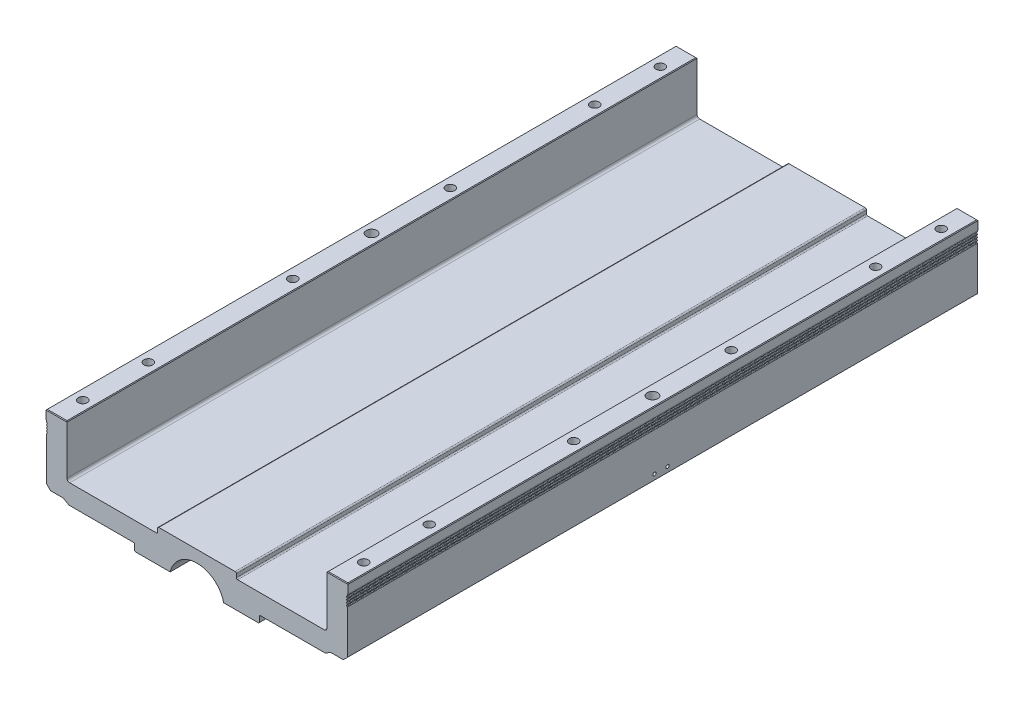
from build123d import *

# Parameters (mm, degrees)
EXTRUDE_1_DEPTH             = 240
CUT_EXTRUDE_1_DEPTH         = 504.178149367
FILLET_1_R                  = 2
FILLET_8_R                  = 1
CUT_EXTRUDE_3_DEPTH         = 504.178149367
FILLET_6_R                  = 0.5
CUT_EXTRUDE_4_DEPTH         = 504.178149367
SKETCH_8_W                  = 1.5
SKETCH_8_H                  = 10.5
CUT_EXTRUDE_6496_DEPTH      = 504.178149367
SKETCH_9_W                  = 230
SKETCH_9_H                  = 1.5
CUT_EXTRUDE_6896_DEPTH      = 503.832974257
SKETCH_10_W                 = 67
SKETCH_10_H                 = 5.5
CUT_EXTRUDE_7625_DEPTH      = 503.832974257
SKETCH_31_W                 = 27
SKETCH_31_H                 = 3
CUT_EXTRUDE_10_DEPTH        = 503.832974257
HOLE_WIZARD_M8_1_D          = 6.8
HOLE_WIZARD_M8_1_DEPTH      = 26.25
HOLE_WIZARD_M8_1_TIP        = 2.042926105
SKETCH_22_R                 = 4
CUT_EXTRUDE_8_DEPTH         = 15
HOLE_WIZARD_M3_1_AT_2_COUNT = 2
HOLE_WIZARD_M3_1_AT_2_PITCH = 10
CHAMFER_3_SIZE              = 0.5
SKETCH_30_R                 = 5
CUT_EXTRUDE_9_DEPTH         = 6
SKETCH_32_W                 = 66
SKETCH_32_H                 = 34.5
CUT_EXTRUDE_11_DEPTH        = 503.832974257


with BuildPart() as part:
    # 草图1 → 凸台-拉伸1 (new, symmetric)
    with BuildSketch(Plane.XY):
        Polygon((-116.5, 0), (116.5, 0), (116.5, -8), (116, -8.5), (114.5, -8.5), (114.5, -50.5), (111.5, -53.5), (101.92820323, -53.5), (95, -57.5), (49, -57.5), (49, -59.5), (47, -61.5), (33, -61.5), (33, -86), (27.226497308, -96), (-27.226497308, -96), (-33, -86), (-33, -61.5), (-47, -61.5), (-49, -59.5), (-49, -57.5), (-95, -57.5), (-101.92820323, -53.5), (-111.5, -53.5), (-114.5, -50.5), (-114.5, -8.5), (-116, -8.5), (-116.5, -8), align=None)
    extrude(amount=EXTRUDE_1_DEPTH, both=True)

    # 草图2 → 切除-拉伸1 (cut, through all)
    with BuildSketch(Plane.XY.offset(240)):
        Polygon((-99, 0), (99, 0), (99, -41), (30, -41), (30, -36.5), (-30, -36.5), (-30, -41), (-99, -41), align=None)
    extrude(amount=-CUT_EXTRUDE_1_DEPTH, mode=Mode.SUBTRACT)

    # 圆角1
    fillet_1_edges = [part.edges().sort_by_distance(p)[0] for p in [
        (99, -41, 0),
        (-99, -41, 0),
    ]]
    fillet(fillet_1_edges, radius=FILLET_1_R)

    # 圆角8
    fillet_8_edges = [part.edges().sort_by_distance(p)[0] for p in [
        (30, -41, 0),
        (30, -36.5, 0),
        (-30, -36.5, 0),
        (-30, -41, 0),
    ]]
    fillet(fillet_8_edges, radius=FILLET_8_R)

    # 草图4 → 切除-拉伸3 (cut, through all)
    with BuildSketch(Plane.XY.offset(240)):
        with BuildLine():
            Line((-114.5, -10), (-114.5, -11))
            ThreePointArc((-114.5, -11), (-114, -10.5), (-114.5, -10))
        make_face()
        with BuildLine():
            Line((-114.5, -12), (-114.5, -13))
            ThreePointArc((-114.5, -13), (-114, -12.5), (-114.5, -12))
        make_face()
        with BuildLine():
            Line((-114.5, -14), (-114.5, -15))
            ThreePointArc((-114.5, -15), (-114, -14.5), (-114.5, -14))
        make_face()
        with BuildLine():
            Line((-114.5, -16), (-114.5, -17))
            ThreePointArc((-114.5, -17), (-114, -16.5), (-114.5, -16))
        make_face()
        with BuildLine():
            Line((114.5, -16), (114.5, -17))
            ThreePointArc((114.5, -17), (114, -16.5), (114.5, -16))
        make_face()
        with BuildLine():
            Line((114.5, -14), (114.5, -15))
            ThreePointArc((114.5, -15), (114, -14.5), (114.5, -14))
        make_face()
        with BuildLine():
            Line((114.5, -12), (114.5, -13))
            ThreePointArc((114.5, -13), (114, -12.5), (114.5, -12))
        make_face()
        with BuildLine():
            Line((114.5, -10), (114.5, -11))
            ThreePointArc((114.5, -11), (114, -10.5), (114.5, -10))
        make_face()
    extrude(amount=-CUT_EXTRUDE_3_DEPTH, mode=Mode.SUBTRACT)

    # 圆角6
    fillet_6_edges = [part.edges().sort_by_distance(p)[0] for p in [
        (-114.5, -14, 0),
        (-114.5, -15, 0),
        (-114.5, -12, 0),
        (-114.5, -13, 0),
        (-114.5, -16, 0),
        (-114.5, -17, 0),
        (-114.5, -10, 0),
        (-114.5, -11, 0),
        (114.5, -13, 0),
        (114.5, -12, 0),
        (114.5, -11, 0),
        (114.5, -10, 0),
        (114.5, -15, 0),
        (114.5, -14, 0),
        (114.5, -17, 0),
        (114.5, -16, 0),
    ]]
    fillet(fillet_6_edges, radius=FILLET_6_R)

    # 草图5 → 切除-拉伸4 (cut, through all)
    with BuildSketch(Plane.XY.offset(240)):
        with BuildLine():
            Line((-13.5, -82.585707942), (-13.5, -93))
            Line((-13.5, -93), (13.5, -93))
            Line((13.5, -93), (13.5, -82.585707942))
            ThreePointArc((13.5, -82.585707942), (0, -45.5), (-13.5, -82.585707942))
        make_face()
    extrude(amount=-CUT_EXTRUDE_4_DEPTH, mode=Mode.SUBTRACT)

    # 草图8 → Cut-Extrude 6496 (cut, through all)
    with BuildSketch(Plane.XY.offset(240)):
        with Locations((115.75, -5.25)):
            Rectangle(SKETCH_8_W, SKETCH_8_H)
        with Locations((-115.75, -5.25)):
            Rectangle(SKETCH_8_W, SKETCH_8_H)
    extrude(amount=-CUT_EXTRUDE_6496_DEPTH, mode=Mode.SUBTRACT)

    # 草图9 → Cut-Extrude 6896 (cut, through all)
    with BuildSketch(Plane.XY.offset(240)):
        with Locations((0, -0.75)):
            Rectangle(SKETCH_9_W, SKETCH_9_H)
    extrude(amount=-CUT_EXTRUDE_6896_DEPTH, mode=Mode.SUBTRACT)

    # 草图10 → Cut-Extrude 7625 (cut, through all)
    with BuildSketch(Plane.XY.offset(240)):
        with Locations((81, -58.75)):
            Rectangle(SKETCH_10_W, SKETCH_10_H)
        with Locations((-81, -58.75)):
            Rectangle(SKETCH_10_W, SKETCH_10_H)
    extrude(amount=-CUT_EXTRUDE_7625_DEPTH, mode=Mode.SUBTRACT)

    # 草图31 → 切除-拉伸10 (cut, through all)
    with BuildSketch(Plane.XY.offset(240)):
        with Locations((0, -94.5)):
            Rectangle(SKETCH_31_W, SKETCH_31_H)
    extrude(amount=-CUT_EXTRUDE_10_DEPTH, mode=Mode.SUBTRACT)

    # M8 螺纹孔1
    with Locations(Plane(origin=(0, -1.5, 0), x_dir=(1, 0, 0), z_dir=(0, 1, 0))):
        with Locations((-107, 60), (-107, -60), (107, -60), (107, 60), (107, 220), (107, -220), (-107, -220), (-107, 220), (107, 170), (107, -170), (-107, -170), (-107, 170)):
            Hole(HOLE_WIZARD_M8_1_D / 2, depth=HOLE_WIZARD_M8_1_DEPTH)
            with Locations((0, 0, -(HOLE_WIZARD_M8_1_DEPTH + HOLE_WIZARD_M8_1_TIP / 2))):  # 118° drill point
                Cone(0, HOLE_WIZARD_M8_1_D / 2, HOLE_WIZARD_M8_1_TIP, mode=Mode.SUBTRACT)

    # 草图22 → 切除-拉伸8 (cut)
    with BuildSketch(Plane(origin=(0, -1.5, 0), x_dir=(1, 0, 0), z_dir=(0, 1, 0))):
        with Locations(Location((-107, 0, 0), (0, 0, 180))):
            Circle(SKETCH_22_R)
        with Locations(Location((107, 0, 0), (0, 0, 180))):
            Circle(SKETCH_22_R)
    extrude(amount=-CUT_EXTRUDE_8_DEPTH, mode=Mode.SUBTRACT)

    # 草图28 → M3 螺纹孔1 (revolve, cut)
    with BuildSketch(Plane(origin=(114.5, -46.5, -4), x_dir=(0, 0, -1), z_dir=(0, 1, 0))):
        Polygon((0, 0), (0, 9.251075774), (1.25, 8.5), (1.25, 0), align=None)
    hole_wizard_m3_1 = revolve(axis=Axis((120.85, -46.5, -4), (-1, 0, 0)), mode=Mode.SUBTRACT)

    # M3 螺纹孔1 at 2: M3 螺纹孔1 ×2
    with Locations(*[(0, 0, i * HOLE_WIZARD_M3_1_AT_2_PITCH) for i in range(1, HOLE_WIZARD_M3_1_AT_2_COUNT)]):
        add(hole_wizard_m3_1, mode=Mode.SUBTRACT)

    # 镜向1: M3 螺纹孔1 across plane
    add(hole_wizard_m3_1.mirror(Plane(origin=(0, 0, 0), x_dir=(0, 0, 1), z_dir=(1, 0, 0))), mode=Mode.SUBTRACT)

    # 镜向1 copy 1 sketch → 镜向1 copy 1 (revolve, cut)
    with BuildSketch(Plane(origin=(-114.5, -46.5, 6), x_dir=(0, 0, -1), z_dir=(0, 1, 0))):
        Polygon((0, 0), (0, -9.251075774), (1.25, -8.5), (1.25, 0), align=None)
    revolve(axis=Axis((-120.85, -46.5, 6), (-1, 0, 0)), mode=Mode.SUBTRACT)

    # 倒角3
    chamfer_3_edges = [part.edges().sort_by_distance(p)[0] for p in [
        (99, -1.5, 0),
        (107, -1.5, -240),
        (115, -1.5, 0),
        (-107, -1.5, -240),
        (-99, -1.5, 0),
        (107, -1.5, 240),
        (-107, -1.5, 240),
        (-115, -1.5, 0),
    ]]
    chamfer(chamfer_3_edges, length=CHAMFER_3_SIZE)

    # 草图30 → 切除-拉伸9 (cut)
    with BuildSketch(Plane.XY.offset(240)):
        with Locations((-26.5, -66.5)):
            Circle(SKETCH_30_R)
        with Locations(Location((26.5, -66.5, 0), (0, 0, 180))):
            Circle(SKETCH_30_R)
    extrude(amount=-CUT_EXTRUDE_9_DEPTH, mode=Mode.SUBTRACT)

    # 草图32 → 切除-拉伸11 (cut, through all)
    with BuildSketch(Plane(origin=(0, 0, -240), x_dir=(-1, 0, 0), z_dir=(0, 0, -1))):
        with Locations((0, -78.75)):
            Rectangle(SKETCH_32_W, SKETCH_32_H)
    extrude(amount=-CUT_EXTRUDE_11_DEPTH, mode=Mode.SUBTRACT)


solid = part.part
